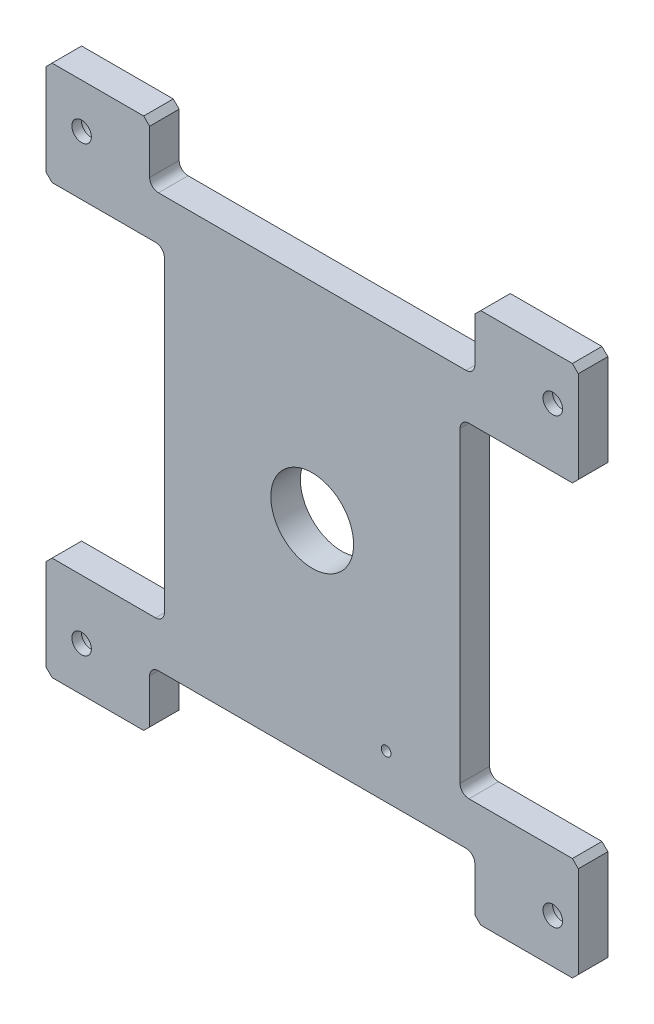
SolidWorks part; units mm, degrees
ref_plane "Front Plane" through (0, 0, 0) normal (0, 0, 1) x (1, 0, 0)
ref_plane "Top Plane" through (0, 0, 0) normal (0, 1, 0) x (1, 0, 0)
ref_plane "Right Plane" through (0, 0, 0) normal (1, 0, 0) x (0, 0, -1)
other "Configuration Table"
sketch "Sketch1" plane through (0, 0, 0) normal (0, 0, 1) x (1, 0, 0)
  line L0 (-90, 55) -> (-50, 55)
  line L5 (-90, -90) -> (-55, -90)
  line L6 (-90, -90) -> (-90, -55)
  line L7 (-90, 90) -> (-55, 90)
  line L8 (90, -90) -> (90, -55)
  line L9 (-90, -90) -> (90, 90) construction
  line L10 (-90, 90) -> (90, -90) construction
  line L11 (-50, 55) -> (-50, -55)
  line L12 (-50, -55) -> (-90, -55)
  line L13 (-90, 55) -> (-90, 90)
  line L14 (0, 0) -> (0, 90) construction
  line L15 (0, 0) -> (50, 0) construction
  line L16 (50, -55) -> (90, -55)
  line L17 (50, 55) -> (50, -55)
  line L18 (90, 55) -> (50, 55)
  line L19 (90, 55) -> (90, 90)
  line L24 (-55, 90) -> (-55, 70)
  line L25 (-55, 70) -> (55, 70)
  line L26 (55, 70) -> (55, 90)
  line L27 (55, -70) -> (55, -90)
  line L28 (-55, -70) -> (55, -70)
  line L29 (-55, -90) -> (-55, -70)
  line L30 (55, -90) -> (90, -90)
  line L31 (55, 90) -> (90, 90)
  point P0 (0, 0)
  dimension "D1" = 180
  dimension "D2" = 180
  dimension "D3" = 35
  dimension "D4" = 35
  dimension "D5" = 40
  dimension "D6" = 35
  dimension "D7" = 20
  dimension "D8" = 35
extrude "Boss-Extrude1" add sketch "Sketch1" along normal blind 10 contours L11 L12 L6 L5 L29 L28 L27 L30 L8 L16 L17 L18 L19 L31 L26 L25 L24 L7 L13 L0
sketch "Sketch2" plane through (0, 0, 0) normal (0, 0, -1) x (-1, 0, 0)
  circle A0 centre (0, 0) radius 14
  dimension "D1" = 28
extrude "Cut-Extrude1" cut sketch "Sketch2" against normal through all
sketch "Sketch3" plane through (0, 0, 10) normal (0, 0, 1) x (1, 0, 0)
hole_wizard "M4 Tapped Hole1" positions "Sketch5" profile "Sketch4" tap size "M4" standard "GB" end condition through all
sketch "Sketch5" plane through (0, 0, 10) normal (0, 0, 1) x (1, 0, 0)
  line L0 (27.5, -55) -> (25, -55) construction
  line L2 (25, -45) -> (25, -55) construction
  line L4 (-55, -70) -> (55, -70) construction
  line L5 (50, 55) -> (50, -55) construction
  point P0 (25, -55)
  dimension "D1" = 2.5
  dimension "D2" = 10
  dimension "D3" = 15
  dimension "D4" = 25
sketch "Sketch4" plane through (25, -55, 10) normal (1, 0, 0) x (0, -1, 0)
  line L0 (0, 0) -> (0, 10)
  line L1 (0, 10) -> (1.65, 10)
  line L2 (1.65, 10) -> (1.65, 0)
  line L5 (1.65, 0) -> (0, 0)
  line L11 (0, -6.35) -> (0, 107.95) construction
  dimension "通孔螺纹孔钻头直径" = 3.3
  dimension "通孔螺纹孔钻头深度" = 10
cosmetic thread "Hole thread line1" parameters "D2"=4
hole_wizard "CBORE for M6 Hexagon socket head cap screws1" positions "Sketch6" profile "Sketch7" counterbore size "M6" standard "GB" end condition through all
sketch "Sketch6" plane through (0, 0, 0) normal (0, 0, -1) x (-1, 0, 0)
  line L0 (0, 0) -> (0, 25.0242) construction
  point P0 (78, -75)
  point P3 (78, 75)
  point P18 (-81.3603, 75)
  point P21 (-81.3603, -75)
sketch "Sketch7" plane through (-78, -75, 0) normal (1, 0, 0) x (0, 1, 0)
  line L0 (0, 0) -> (0, 10)
  line L1 (0, 10) -> (3.3, 10)
  line L3 (3.3, 10) -> (3.3, 6.8)
  line L4 (3.3, 6.8) -> (5.5, 6.8)
  line L5 (5.5, 6.8) -> (5.5, 0)
  line L7 (5.5, 0) -> (0, 0)
  line L11 (0, -6.35) -> (0, 107.95) construction
  dimension "通孔孔直径" = 6.6
  dimension "通孔孔深度" = 10
  dimension "柱形沉头孔直径" = 11
  dimension "柱形沉头孔深度" = 6.8
chamfer "Chamfer1" distance 2 angle 45 12 edges at (-90, 55, 5) (90, 55, 5) (90, -55, 5) (55, -90, 5) (90, -90, 5) (-55, -90, 5) (-90, -90, 5) (-90, -55, 5) (55, 90, 5) (-55, 90, 5) (-90, 90, 5) (90, 90, 5)
fillet "Fillet1" radius 3 8 edges at (50, 55, 5) (50, -55, 5) (55, -70, 5) (55, 70, 5) (-55, 70, 5) (-55, -70, 5) (-50, -55, 5) (-50, 55, 5)
